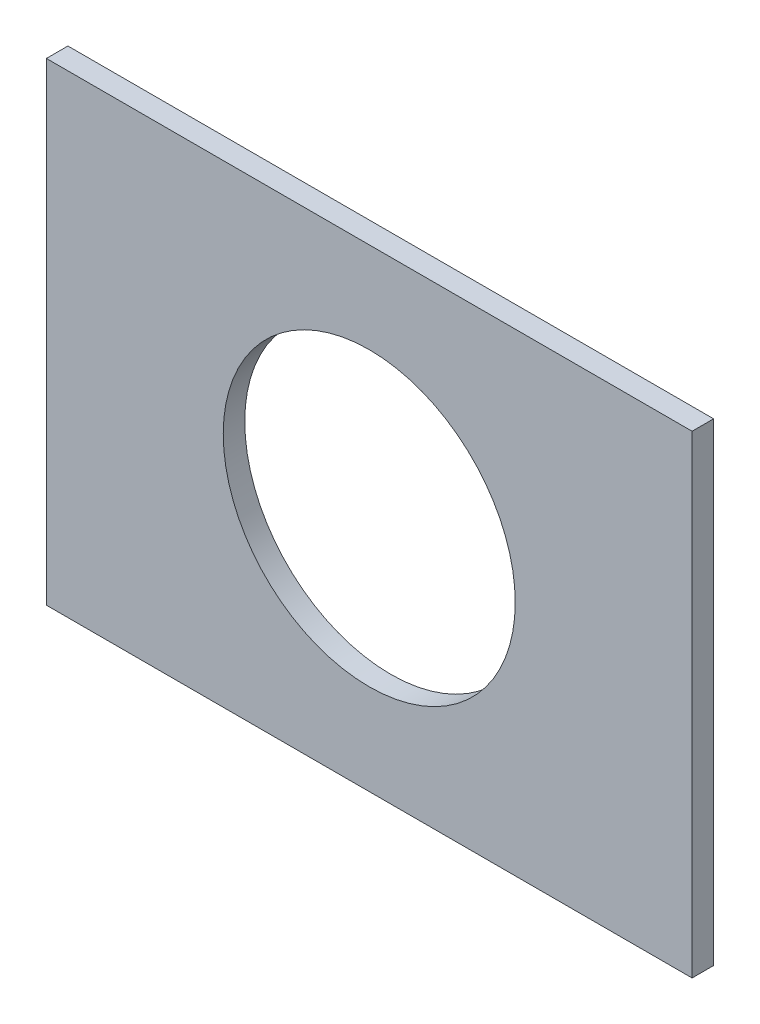
SolidWorks part; units mm, degrees
material "1023 碳钢板 (SS)"
ref_plane "前视基准面" through (0, 0, 0) normal (0, 0, 1) x (1, 0, 0)
ref_plane "上视基准面" through (0, 0, 0) normal (0, 1, 0) x (1, 0, 0)
ref_plane "右视基准面" through (0, 0, 0) normal (1, 0, 0) x (0, 0, -1)
sketch "草图1" plane through (0, 0, 0) normal (0, 0, 1) x (1, 0, 0)
  line L1 (75, -55) -> (-75, -55)
  line L2 (75, -55) -> (75, 55)
  line L3 (75, 55) -> (-75, 55)
  line L4 (-75, -55) -> (-75, 55)
  line L5 (75, -55) -> (-75, 55) construction
  line L6 (75, 55) -> (-75, -55) construction
  point P0 (0, 0)
  dimension "D1" = 110
  dimension "D2" = 150
extrude "凸台-拉伸1" add sketch "草图1" along normal mid plane 5
sketch "草图2" plane through (0, 0, -2.5) normal (0, 0, -1) x (-1, 0, 0)
  line L1 (75, 55) -> (75, -55) construction
  circle A0 centre (0, 0) radius 33.9159
  dimension "D1" = 75
extrude "切除-拉伸1" cut sketch "草图2" against normal blind 10
